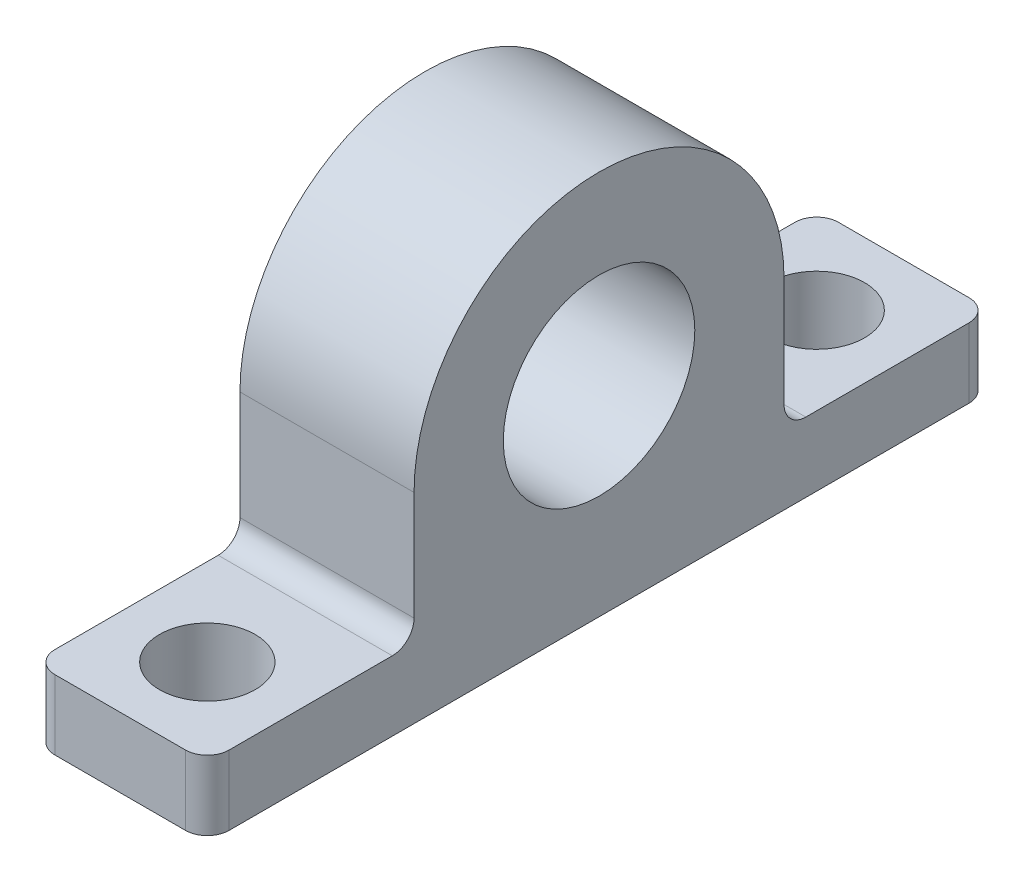
SolidWorks part; units mm, degrees
material "普通碳钢"
ref_plane "Front Plane" through (0, 0, 0) normal (0, 0, 1) x (1, 0, 0)
ref_plane "Top Plane" through (0, 0, 0) normal (0, 1, 0) x (1, 0, 0)
ref_plane "Right Plane" through (0, 0, 0) normal (1, 0, 0) x (0, 0, -1)
sketch "Sketch1" plane through (0, 0, 0) normal (0, 1, 0) x (1, 0, 0)
  line L0 (0, 90) -> (0, 0) construction
  line L1 (-20, 90) -> (20, 90)
  line L2 (-20, 90) -> (-20, -90)
  line L3 (-20, -90) -> (20, -90)
  line L4 (20, 90) -> (20, -90)
  line L5 (0, 0) -> (-20, 0) construction
  circle A0 centre (0, 70) radius 11
  circle A1 centre (0, -70) radius 11
  dimension "D3" = 22
  dimension "D1" = 180
  dimension "D2" = 40
  dimension "D4" = 140
extrude "Boss-Extrude1" add sketch "Sketch1" along normal blind 16
sketch "Sketch2" plane through (0, 0, 0) normal (1, 0, 0) x (0, 0, -1)
  line L0 (0, 22) -> (0, -22) construction
  line L1 (-42.5, 46) -> (-42.5, 16)
  line L2 (-90, 16) -> (90, 16) construction
  line L3 (42.5, 46) -> (42.5, 16)
  line L4 (-42.5, 16) -> (42.5, 16)
  circle A0 centre (0, 46) radius 22
  arc A1 (42.5, 46) -> (-42.5, 46) centre (0, 46) ccw
  dimension "D2" = 44
  dimension "D3" = 30
  dimension "D1" = 85
extrude "Boss-Extrude2" add sketch "Sketch2" along normal mid plane 40
fillet "Fillet1" radius 5 6 edges at (20, 8, 90) (-20, 8, 90) (20, 8, -90) (-20, 8, -90)
